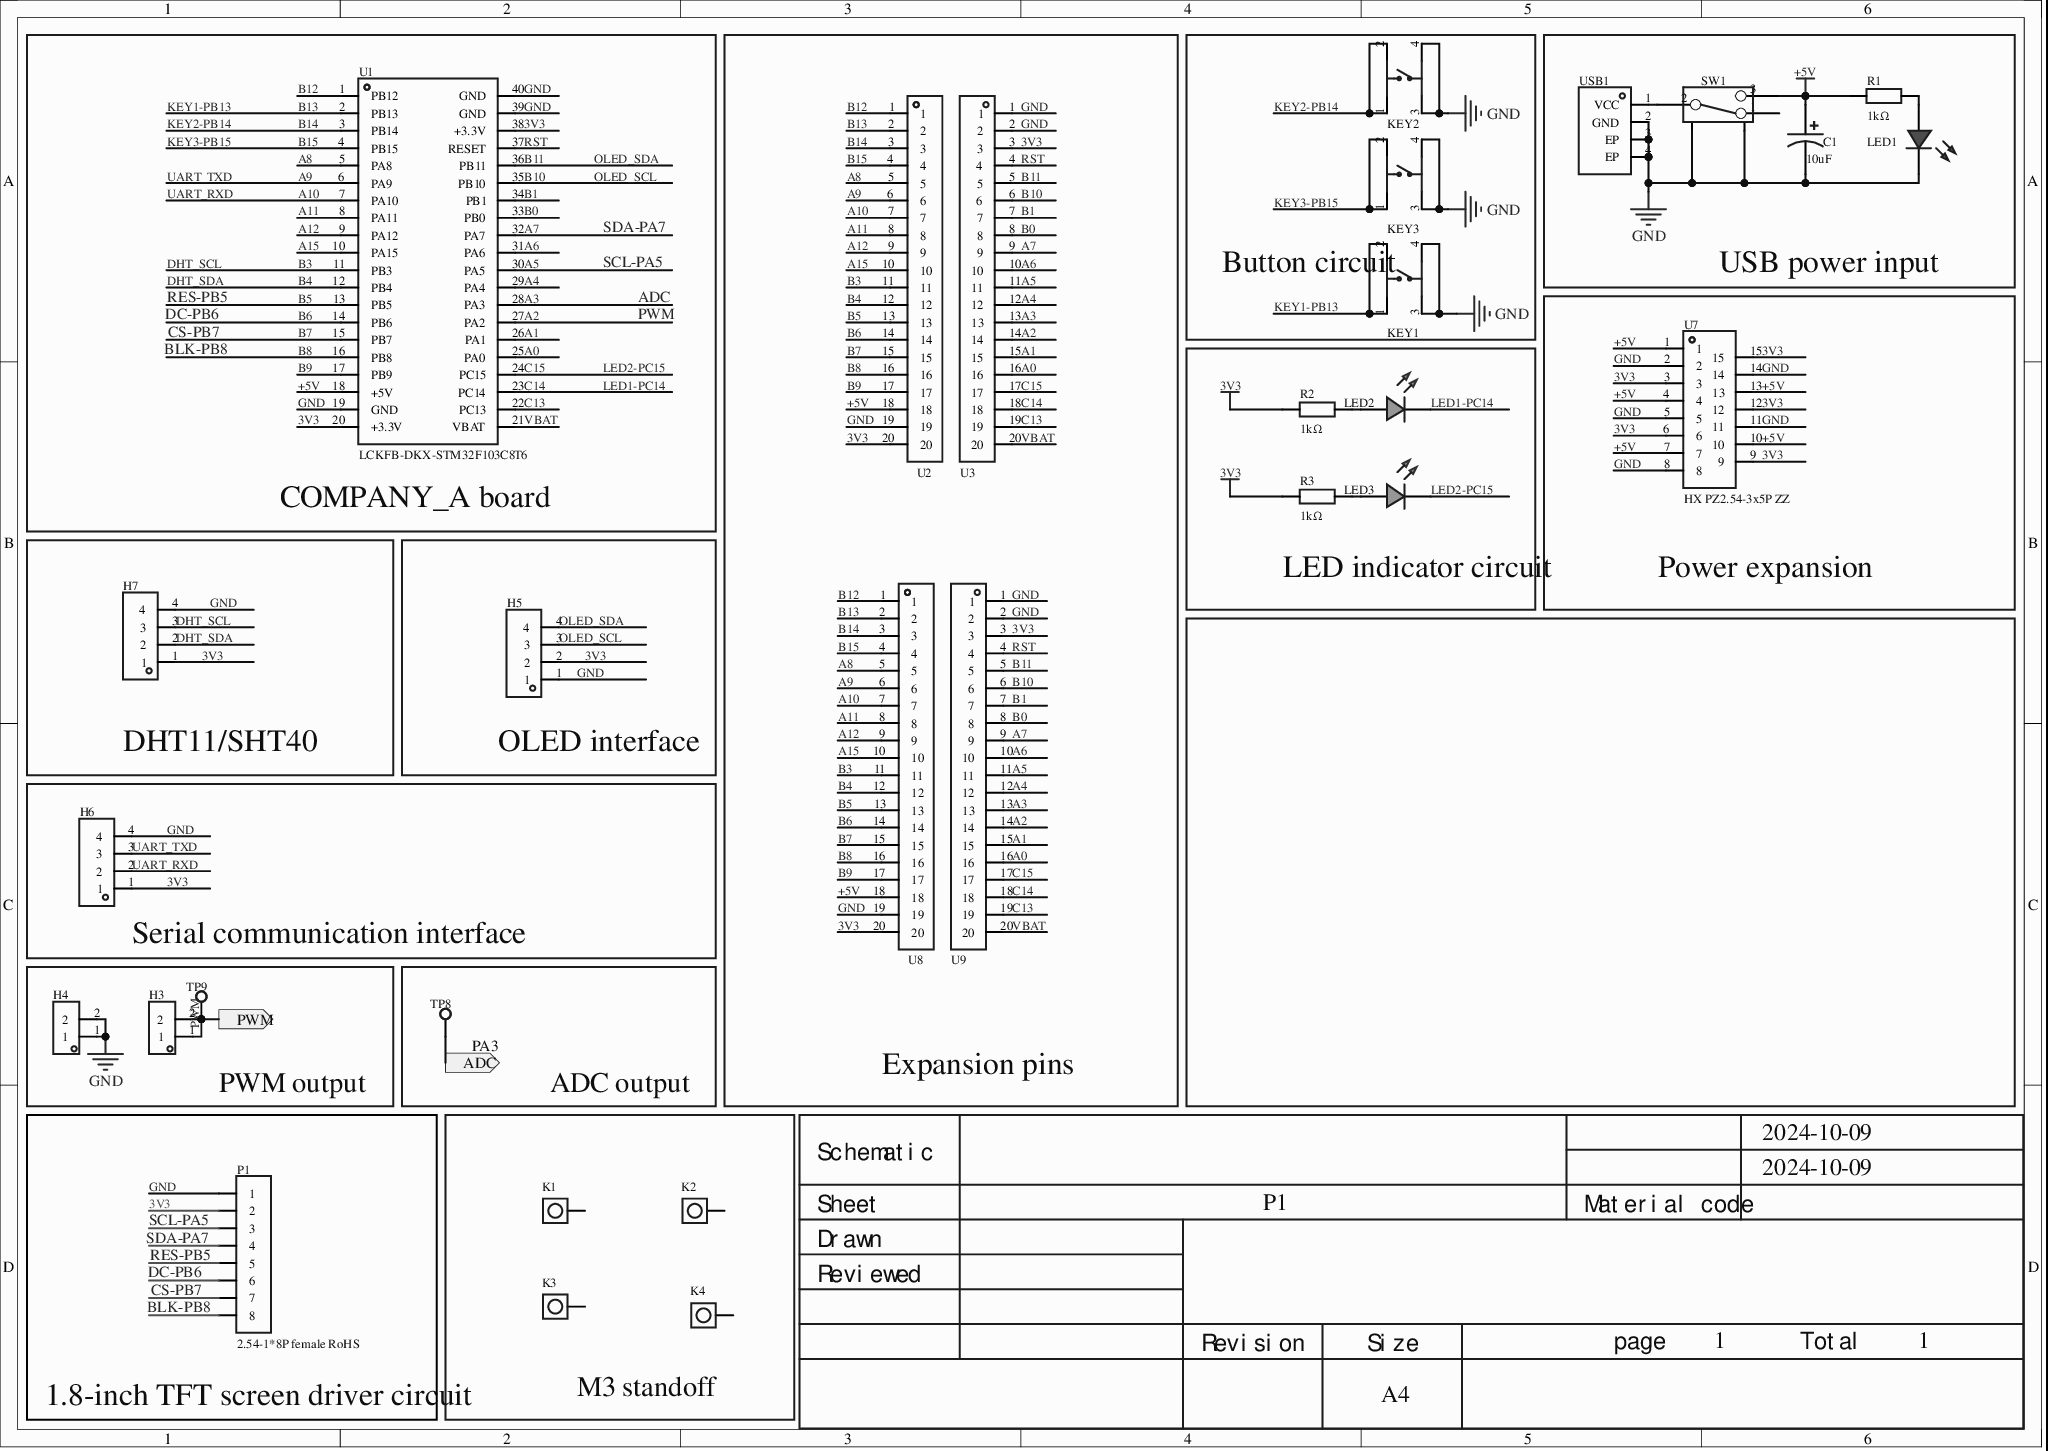
[diagram p0: MISC75409-3.schdoc]
# Altium project MISC75409-2.PrjPcb
1 sheet, 30 parts. Net scope: flat (ports and power ports of the same name join across sheets).
Board file: MISC75409.pcbdoc

## Sheet MISC75409-3.schdoc
size 297 x 210 mm; Version: V1.0; @Project Name: MISC75409; @Page Count: 1; @Update Date: 2024-10-09; @Create Date: 2024-10-09; @Schematic Name: MISC75409; @Page No: 1; @Board Name: MISC75409; @Create Time: 20:43:25; @Update Time: 20:43:25

### Parts
C1  value 10uF  [CAP-TH_BD5.0-P2.00-D0.8-FD]  (hidden comment: 01EC1809SHC10UF50V)
H3  HDR-M_2.54_1x2P  [HDR-TH_2P-P2.54-V-M-1]  (value not drawn)
H4  HDR-M_2.54_1x2P  [HDR-TH_2P-P2.54-V-M-1]  (value not drawn)
H5  2.54-1*4P female  [HDR-TH_4P-P2.54-V-F]  (value not drawn)
H6  2.54-1*4P female  [HDR-TH_4P-P2.54-V-F]  (value not drawn)
H7  2.54-1*4P female  [HDR-TH_4P-P2.54-V-F]  (value not drawn)
K1  Flange pad  [法兰焊盘-8孔-M3]  (value not drawn)
K2  Flange pad  [法兰焊盘-8孔-M3]  (value not drawn)
K3  Flange pad  [法兰焊盘-8孔-M3]  (value not drawn)
K4  Flange pad  [法兰焊盘-8孔-M3]  (value not drawn)
KEY1  TC-6610-9-260G  [SW-TH_4P-L5.0-W5.0-P4.50-LS6.5]  (value not drawn)
KEY2  TC-6610-9-260G  [SW-TH_4P-L5.0-W5.0-P4.50-LS6.5]  (value not drawn)
KEY3  TC-6610-9-260G  [SW-TH_4P-L5.0-W5.0-P4.50-LS6.5]  (value not drawn)
LED1  LED_TH-R_3mm  [LED_TH-3mm]  (value not drawn)
LED2  LED_TH-G_3mm  [LED_TH-3mm]  (value not drawn)
LED3  LED_TH-G_3mm  [LED_TH-3mm]  (value not drawn)
P1  2.54-1*8P female RoHS  [HDR-TH_8P-P2.54-V-F-1]
R1  value 1kΩ  [RES-TH_BD2.5-L6.5-P10.50-D0.6]  (hidden comment: MFR0W4F1001A50)
R2  value 1kΩ  [RES-TH_BD2.5-L6.5-P10.50-D0.6]  (hidden comment: MFR0W4F1001A50)
R3  value 1kΩ  [RES-TH_BD2.5-L6.5-P10.50-D0.6]  (hidden comment: MFR0W4F1001A50)
SW1  SK-12E12-G5  [SW-TH_SK-12E12-G5]  (value not drawn)
TP8  TP-yellow test point  [TESTPOINT-TH_BD3.2]  (value not drawn)
TP9  TP-yellow test point  [TESTPOINT-TH_BD3.2]  (value not drawn)
U1  LCKFB-DKX-STM32F103C8T6  [CONN-TH_L53.3-W22.9_STM32F103C8T6-CARD]
U2  KH-2.54FH-1X20P-H8.5  [HDR-TH_20P-P2.54-V-F-2]  (value not drawn)
U3  KH-2.54FH-1X20P-H8.5  [HDR-TH_20P-P2.54-V-F-2]  (value not drawn)
U7  HX PZ2.54-3x5P ZZ  [HDR-TH_15P-P2.54-V-M-R3-C5-S7.5]
U8  KH-2.54FH-1X20P-H8.5  [HDR-TH_20P-P2.54-V-F-2]  (value not drawn)
U9  KH-2.54FH-1X20P-H8.5  [HDR-TH_20P-P2.54-V-F-2]  (value not drawn)
USB1  KH-TYPE-C-2P  [USB-SMD_KH-TYPE-C-2P]  (value not drawn)

### Blocks framed on the sheet
COMPANY_A board: U1
Expansion pins: U2 U3 U8 U9
Button circuit: KEY1-KEY3
USB power input: C1 LED1 R1 SW1 USB1
Power expansion: U7
LED indicator circuit: LED2 LED3 R2 R3
DHT11/SHT40: H7
OLED interface: H5
Serial communication interface: H3 H4 TP9
ADC output: TP8
1.8-inch TFT screen driver circuit: P1
M3 standoff: K1-K4

### Ports
ADC (out), PWM (out)

### Nets
3V3: H5.2 H6.1 H7.1 P1.2 R2.2 R3.2 U1.20(+3.3V) U1.38(+3.3V) U2.20 U3.3 U7.3 U7.6 U7.9 U7.12 U7.15 U8.20 U9.3
+5V: C1.1 R1.2 SW1.3 U1.18(+5V) U2.18 U7.1 U7.4 U7.7 U7.10 U7.13 U8.18
GND: C1.2 H4.1 H4.2 H5.1 H6.4 H7.4 KEY1.3 KEY1.4 KEY2.3 KEY2.4 KEY3.3 KEY3.4 LED1.2(A) P1.1 SW1.4 SW1.5 U1.19(GND) U1.39(GND) U1.40(GND) U2.19 U3.1 U3.2 U7.2 U7.5 U7.8 U7.11 U7.14 U8.19 U9.1 U9.2 USB1.2(GND) USB1.3(EP) USB1.4(EP)
A0: U1.25(PA0) U3.16 U9.16
A1: U1.26(PA1) U3.15 U9.15
A2: H3.1 H3.2 TP9.1 U1.27(PA2) U3.14 U9.14 ; port PWM  [also labelled PWM]
A3: U1.28(PA3) U3.13 U9.13  [also labelled ADC]
A4: U1.29(PA4) U3.12 U9.12
A5: P1.3 U1.30(PA5) U3.11 U9.11  [also labelled SCL-PA5]
A6: U1.31(PA6) U3.10 U9.10
A7: P1.4 U1.32(PA7) U3.9 U9.9  [also labelled SDA-PA7]
A8: U1.5(PA8) U2.5 U8.5
A9: H6.3 U1.6(PA9) U2.6 U8.6  [also labelled UART_TXD]
A10: H6.2 U1.7(PA10) U2.7 U8.7  [also labelled UART_RXD]
A11: U1.8(PA11) U2.8 U8.8
A12: U1.9(PA12) U2.9 U8.9
A15: U1.10(PA15) U2.10 U8.10
B0: U1.33(PB0) U3.8 U9.8
B1: U1.34(PB1) U3.7 U9.7
B3: H7.3 U1.11(PB3) U2.11 U8.11  [also labelled DHT_SCL]
B4: H7.2 U1.12(PB4) U2.12 U8.12  [also labelled DHT_SDA]
B5: P1.5 U1.13(PB5) U2.13 U8.13  [also labelled RES-PB5]
B6: P1.6 U1.14(PB6) U2.14 U8.14  [also labelled DC-PB6]
B7: P1.7 U1.15(PB7) U2.15 U8.15  [also labelled CS-PB7]
B8: P1.8 U1.16(PB8) U2.16 U8.16  [also labelled BLK-PB8]
B9: U1.17(PB9) U2.17 U8.17
B10: H5.3 U1.35(PB10) U3.6 U9.6  [also labelled OLED_SCL]
B11: H5.4 U1.36(PB11) U3.5 U9.5  [also labelled OLED_SDA]
B12: U1.1(PB12) U2.1 U8.1
B13: KEY1.1 KEY1.2 U1.2(PB13) U2.2 U8.2  [also labelled KEY1-PB13]
B14: KEY2.1 KEY2.2 U1.3(PB14) U2.3 U8.3  [also labelled KEY2-PB14]
B15: KEY3.1 KEY3.2 U1.4(PB15) U2.4 U8.4  [also labelled KEY3-PB15]
C13: U1.22(PC13) U3.19 U9.19
C14: LED2.2(A) U1.23(PC14) U3.18 U9.18  [also labelled LED1-PC14]
C15: LED3.2(A) U1.24(PC15) U3.17 U9.17  [also labelled LED2-PC15]
RST: U1.37(RESET) U3.4 U9.4
VBAT: U1.21(VBAT) U3.20 U9.20
NetLED1_1: LED1.1(C) R1.1
NetLED2_1: LED2.1(C) R2.1
NetLED3_1: LED3.1(C) R3.1
NetSW1_2: SW1.2 USB1.1(VCC)
NetTP8_1: TP8.1 ; port ADC

Not connected (* = marked no-connect by the designer): K1 1; K2 1; K3 1; K4 1; SW1 1*

### Notes on the sheet
- (near TP8) PA3
- PWM output
- 2024-10-09
- Schematic
- Sheet
- P1
- Material code
- Reviewed
- Drawn
- Revision
- Size
- A4
- page
- 1
- Total

### Library data of the parts
C1 = 01EC1809SHC10UF50V: Capacitance: 10uF; tolerance: ±20%; rated voltage: 50V; ripple current: 50mA@120Hz; ESR: -;; Manufacturer: KNSCHA(科尼盛); AddInBom: yes; ModelId: edeeed87cbc746108d01291548c38636; ModelName: CAP-TH_D5.0×H7.0×P2.0; ModelTransform: 197.091,196.7911,0,0,0,0,0,0,-137.795; φD: 5mm; L: 11mm; Lifetime @ Temp: 5000hrs@105℃; Symbol: 01EC1809SHC10UF50V; Device: 01EC1809SHC10UF50V; Supplier: LCSC; Supplier Part: C503219; Manufacturer Part: 01EC1809SHC10UF50V; JLCPCB Part Class: Extended library; LCSC Part Name: 10uF ±20% 50V; Supplier Footprint: 插件,D5xL11mm; Datasheet: https://atta.szlcsc.com/upload/public/pdf/source/20200324/C503219_39D1683F20D4DB1C41D8BE9142629697.pdf; ConvertToPcb: yes; FootprintName: CAP-TH_BD5.0-P2.00-D0.8-FD; Tolerance: ±20%; Rated Voltage: 50V; Ripple Current: 50mA@120Hz; Equivalent Series Resistance(ESR): -; Lead Spacing: 2mm
H3 H4 = HDR-M_2.54_1x2P: ConvertToPcb: yes; SymbolName: 210S-1*2P L=11.6MMGold-plated black; ModelId: 79b2e9f2d70a4d68a1b7098f27c6d4c5; ModelName: HDR-M-2.54_1x2; ModelTransform: 200,100,0,0,0,0,0,0,-118.11; Device: HDR-M_2.54_1x2P; AddInBom: yes; SupplierPart: C124375; Supplier Footprint: 插件; FootprintName: HDR-TH_2P-P2.54-V-M-1
H5-H7 = 2.54-1*4P母: Socket structure: 1x4P; pitch: 2.54mm; row spacing: -; round/square hole: square hole; mounting type: through-hole; rows: single row; total positions: 4P; rated current: 3A; rated voltage: -; socket direction: top; height: -; contact material: bronze; contact plating: -; operating temperature: -40℃~+105℃; soldering temperature (max): -;; Manufacturer: BOOMELE(博穆精密); AddInBom: yes; ModelId: 57daaad411c24bd7bd5d06edf5c4d16b; ModelName: HDR-TH_4P-P2.54-F-LI-1X4P; ModelTransform: 415.7472,98.425,0,0,0,0,0,0,-118.11; Symbol: 2.54-1*4P female; Device: 2.54-1*4P female; Supplier: LCSC; Supplier Part: C2718488; Manufacturer Part: 2.54-1*4P母; JLCPCB Part Class: Extended library; LCSC Part Name: 间距:2.54mm 1x4P 直插; Supplier Footprint: 插件,P=2.54mm; Datasheet: https://atta.szlcsc.com/upload/public/pdf/source/20210301/C2718488_F4427B881E42CAA8DDB0B1C12B3A522C.pdf; ConvertToPcb: yes; FootprintName: HDR-TH_4P-P2.54-V-F; Holes Structure: 1x4P; Pitch: 2.54mm; Row Spacing: -; Circular Hole / Square Hole: Square hole; Mounting Type: Through-hole; Number of Rows: Single row; Number of Holes: 4P; Current Rating (Max): 3A; Voltage Rating (Max): -; Holes Direction: Top; Insulation Height: -; Contact Material: Bronze; Contact Plating: -; Operating Temperature Range: -40℃~+105℃; Soldering Temperature(Max): -
K1-K4 = 法兰焊盘-8孔-M3: ConvertToPcb: yes; Device: 法兰焊盘-8孔-M3; AddInBom: yes; SymbolName: 法兰焊盘-8孔-M3; FootprintName: 法兰焊盘-8孔-M3
KEY1-KEY3 = TC-6610-9-260G: Contact current: 50mA; rated voltage (AC): -; rated voltage (DC): 12V; rated power: -; insulation resistance: -; circuit: SPST; mounting style: upright SMD; with LED: -; actuating force: -; mechanical life: 10 wan cycles; with bracket: No;; Manufacturer: HCTL(华灿天禄); AddInBom: yes; ModelId: 98d777fa0d8e4b349f8964973a43b5c6; ModelTransform: 298.97956,196.85,0,0,0,0,0,0,-98.425; Actuator Style: Round button; Actuator/Cap Color: Black; Pin Style: Gull-wing; Switch Length: 6mm; Switch Height: 9mm; Device: TC-6610-9-260G; Symbol: TC-6610-9-260G; LCSC Part Name: 6*6*9mm 立贴 轻触开关; SupplierPart: C2845257; ManufacturerPart: TC-6610-9-260G; Supplier Footprint: 插件; JLCPCB Part Class: Extended library; Datasheet: https://atta.szlcsc.com/upload/public/pdf/source/20230323/2FDB5D6FCE87B7593CD3E5FAC75F65D7.pdf; Supplier: LCSC; ConvertToPcb: yes; FootprintName: SW-TH_4P-L5.0-W5.0-P4.50-LS6.5; ModelName: SW-TH_4P-L5.0-W5.0-P4.50-LS6.5; Contact Current: 50mA; Voltage Rating (AC): -; Voltage Rating (DC): 12V; Power Rating: -; Insulation Resistance: -; Circuit: SPST; Mounting Style: Upright SMD; With Lamp: -; Operating Force: -; Mechanical Life: 10 wan cycles; Operating Temperature: -; IP Rating: -; Diameter: -; Switch Width: 6mm; Strike Gundam: No
LED1 = LED_TH-R_3mm: ConvertToPcb: yes; ModelId: a497c992633541038a38947cdc58012f; ModelName: LED-TH-3mm_R; ModelTransform: 141.274,153.327,0,0,0,0,-5.984,0,-137.795; Symbol: LED_TH-R; Device: LED_TH-R_3mm; Supplier: 立创商城; Supplier Part: C2895470; AddInBom: yes; FootprintName: LED_TH-3mm; Supplier Footprint: 插件
LED2 LED3 = LED_TH-G_3mm: ConvertToPcb: yes; ModelId: a497c992633541038a38947cdc58012f; ModelName: LED-TH-3mm_R; ModelTransform: 141.274,153.327,0,0,0,0,-5.984,0,-137.795; Device: LED_TH-G_3mm; Supplier Part: C2895477; Supplier: 立创商城; AddInBom: yes; SymbolName: LED_TH-G; FootprintName: LED_TH-3mm; Supplier Footprint: 插件
P1 = 2.54-1*8P母环保: Socket structure: 1x8P; pitch: 2.54mm; row spacing: -; mounting type: through-hole; rows: single row; total positions: 8P; height: -; contact material: -; contact plating: -;; Manufacturer: BOOMELE(博穆精密); Symbol: Header-Female-2.54_1x8; AddInBom: yes; ModelId: 0f7e4d9227ef4fa08d5469c22cc70cdb; ModelName: HDR-F-2.54_1x8; ModelTransform: 799.99844,100,0,0,0,0,0,0,-118.11; Device: 2.54-1*8P female RoHS; Supplier: LCSC; Manufacturer Part: 2.54-1*8P母环保; Supplier Part: C27438; JLCPCB Part Class: Extended library; LCSC Part Name: 间距:2.54mm 1x8P 直插; Supplier Footprint: 插件,P=2.54mm; Datasheet: https://atta.szlcsc.com/upload/public/pdf/source/20231221/1CA800C6799ED97958773716FAA1BFFE.pdf; ConvertToPcb: yes; FootprintName: HDR-TH_8P-P2.54-V-F-1; Holes Structure: 1x8P; Pitch: 2.54mm; Row Spacing: -; Mounting Type: Through-hole; Number of Rows: Single row; Number of Holes: 8P; Insulation Height: -; Contact Material: -; Contact Plating: -
R1-R3 = MFR0W4F1001A50: Resistor type: metal film resistor; resistance: 1kΩ; tolerance: ±1%; power: 250mW; temperature coefficient: ±50ppm/℃;; Manufacturer: UNI-ROYAL(厚声); AddInBom: yes; ModelId: 8e6c7ee8323443d1ab8f0504b6353c8c; ModelName: RES-TH_D2.3-L6.5-P10.50; ModelTransform: 431.1015,91.3384,0,0,0,0,0.197,0,-137.795; Device: MFR0W4F1001A50; Symbol: MFR0W4F1001A50; LCSC Part Name: 金属膜电阻 1kΩ ±1% 250mW; SupplierPart: C57435; ManufacturerPart: MFR0W4F1001A50; Supplier Footprint: 轴向引线; JLCPCB Part Class: Extended library; Datasheet: https://atta.szlcsc.com/upload/public/pdf/source/20170615/1497511028539.pdf; Supplier: LCSC; ConvertToPcb: yes; FootprintName: RES-TH_BD2.5-L6.5-P10.50-D0.6; Type: Metal film resistor; Tolerance: ±1%; Power(Watts): 250mW; Temperature Coefficient: ±50ppm/℃
SW1 = SK-12E12-G5: Rated current (DC): -; rated voltage (DC): -; rated current (AC): -; rated voltage (AC): -; circuit: SPDT; mounting style: horizontal insertion; mechanical life: 5 thousand cycles;; Manufacturer: 韩国韩荣; AddInBom: yes; ModelId: 63ecb7c3b60e41c79481f203e3e77e6b; ModelTransform: 507.874,401.575,0,90,0,0,105,0,-137.795; Actuator Style: Rectangular column; Pin Style: PC pins; Switch Height: 10.6mm; Device: SK-12E12-G5; Symbol: SK-12E12-G5; LCSC Part Name: 卧插双档 滑动开关; SupplierPart: C136720; ManufacturerPart: SK-12E12-G5; Supplier Footprint: 插件; JLCPCB Part Class: Extended library; Datasheet: https://atta.szlcsc.com/upload/public/pdf/source/20210810/880D64C2F8CCE477762EFCC00B7B7681.pdf; Supplier: LCSC; ConvertToPcb: yes; FootprintName: SW-TH_SK-12E12-G5; ModelName: SW-TH_SK-12E12-G5; Current Rating (DC): -; Voltage Rating (DC): -; Current Rating (AC): -; Voltage Rating (AC): -; Circuit: SPDT; Mounting Style: Horizontal insertion; Mechanical Life: 5 thousand cycles; Operating Temperature: -25℃~+70℃
TP8 TP9 = TP-黄色测试点: Add into BOM: no; ConvertToPcb: yes; ModelId: 6bb19dcb8ff8413ea73fe7a5b79be1e3; ModelTransform: 125.984,125.84132,0,0,0,0,0,0,-125.984; Device: TP-yellow test point; LCSC Part Name: TP-黄色测试点; SupplierPart: C9900007422; ManufacturerPart: TP-黄色测试点; Supplier Footprint: TESTPOINT-TH_BD-2P-P2.00; JLCPCB Part Class: Extended library; Supplier: LCSC; SymbolName: TP-yellow test point; FootprintName: TESTPOINT-TH_BD3.2; ModelName: TESTPOINT-TH_BD3.2
U1 = LCKFB-DKX-STM32F103C8T6: Manufacturer: 立创开发板; AddInBom: yes; Symbol: LCKFB-DKX-STM32F103C8T6; Device: LCKFB-DKX-STM32F103C8T6; LCSC Part Name: 立创·地阔星-STM32F103C8T6开发板; SupplierPart: C22396880; ManufacturerPart: LCKFB-DKX-STM32F103C8T6; Supplier Footprint: -; Datasheet: https://atta.szlcsc.com/upload/public/pdf/source/20240801/7EEF69F7480DF7C6DA98696664D658D4.pdf; Supplier: LCSC; ConvertToPcb: yes; FootprintName: CONN-TH_L53.3-W22.9_STM32F103C8T6-CARD
U2 U3 U8 U9 = KH-2.54FH-1X20P-H8.5: Socket structure: 1x20P; pitch: 2.54mm; row spacing: -; round/square hole: square hole; mounting type: through-hole; rows: single row; total positions: 20P; rated current: 3A; rated voltage: -; socket direction: top; height: 8.5mm; operating temperature: -40℃~+105℃;; Manufacturer: kinghelm(金航标); AddInBom: yes; ModelId: 48d3332f1f604cb48783c9ca75931f3b; ModelTransform: 1999.996,98.8187,0,0,0,0,0,0,-106.299; Symbol: KH-2.54FH-1X20P-H8.5; Device: KH-2.54FH-1X20P-H8.5; Supplier: LCSC; Supplier Part: C2905423; Manufacturer Part: KH-2.54FH-1X20P-H8.5; JLCPCB Part Class: Extended library; LCSC Part Name: 间距:2.54mm 1x20P 直插; Supplier Footprint: 插件,P=2.54mm; Datasheet: https://atta.szlcsc.com/upload/public/pdf/source/20211019/BDB673907948473CE61C8A1CF06C5BF5.pdf; ConvertToPcb: yes; FootprintName: HDR-TH_20P-P2.54-V-F-2; ModelName: HDR-TH_20P-P2.54-V-F-2; Holes Structure: 1x20P; Pitch: 2.54mm; Row Spacing: -; Circular Hole / Square Hole: Square hole; Mounting Type: Through-hole; Number of Rows: Single row; Number of Holes: 20P; Current Rating (Max): 3A; Voltage Rating (Max): -; Holes Direction: Top; Insulation Height: 8.5mm; Operating Temperature Range: -40℃~+105℃
U7 = HX PZ2.54-3x5P ZZ: Pin structure: 3x5P; pitch: 2.54mm; row spacing: -; round/square pin: square pin; mounting type: through-hole; rows: three rows; total pins: 15P; rated current: 3A; rated voltage: 1kV; mating pin length: 3mm; height: 2.5mm; tail length: 6mm; contact material: brass; contact plating: gold; operating temperature: -40℃~+105℃; soldering temperature (max): 260℃;; Manufacturer: hanxia(韩下); AddInBom: yes; ModelId: 689266d4928c4af69e39b256dd02c5f1; ModelTransform: 500.3927,295.275,0,0,0,0,0,0,-118.11; Symbol: hx pz2.54-3x5p zz; Device: HX PZ2.54-3x5P ZZ; LCSC Part Name: 3x5P 间距:2.54mm 方针 直插; SupplierPart: C32713292; ManufacturerPart: HX PZ2.54-3x5P ZZ; Supplier Footprint: 插件,P=2.54mm; JLCPCB Part Class: Extended library; Datasheet: https://atta.szlcsc.com/upload/public/pdf/source/20240723/775D0BCA343D2E9C3C7985AB6A29A27A.pdf; Supplier: LCSC; ConvertToPcb: yes; FootprintName: HDR-TH_15P-P2.54-V-M-R3-C5-S7.5; ModelName: HDR-TH_15P-P2.54-V-M-R3-C5-S7.5; Pin Structure: 3x5P; Pitch: 2.54mm; Row Spacing: -; Circluar Pins/Square Pins: Square pin; Mounting Type: Through-hole; Number of Rows: Three rows; Number of Pins: 15P; Current Rating (Max): 3A; Voltage Rating (Max): 1kV; Length of Mating Pin: 3mm; Insulation Height: 2.5mm; Length of End Connection Pin: 6mm; Contact Material: Brass; Contact Plating: Gold; Operating Temperature Range: -40℃~+105℃; Soldering Temperature(Max): 260℃
USB1 = KH-TYPE-C-2P: Connector type: -; standard: -; male/female: -; number of contacts: -; number of ports: -; mounting type: -; rated current - power: -; contact material: -; contact plating: -; operating temperature range: -;; Manufacturer: kinghelm(金航标); AddInBom: yes; ModelId: 4464b34a7d0f48c2b8c2350e914c93f5; ModelTransform: 352.362,255.31449,0,0,0,0,0,-49.213,-98.425; Symbol: KH-TYPE-C-2P; Device: KH-TYPE-C-2P; Supplier: LCSC; Supplier Part: C2919656; Manufacturer Part: KH-TYPE-C-2P; JLCPCB Part Class: Extended library; LCSC Part Name: KH-TYPE-C-2P; Supplier Footprint: 插件; Datasheet: https://atta.szlcsc.com/upload/public/pdf/source/20220707/620587A9E0589B27D96D3CEE595CBC98.pdf; ConvertToPcb: yes; FootprintName: USB-SMD_KH-TYPE-C-2P; ModelName: USB-SMD_KH-TYPE-C-2P; Connector Type: -; Standard: -; Gender: -; Number of Contacts: -; Number of Ports: -; Mounting Style: -; Current Rating - Power (Max): -; Contact Material: -; Contact Plating: -; Operating Temperature Range: -